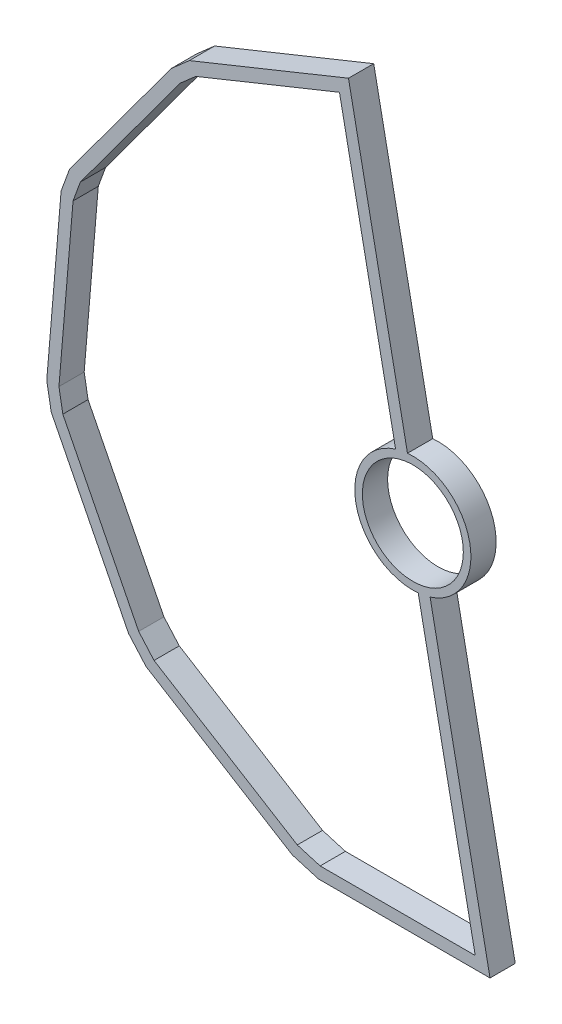
SolidWorks part; units mm, degrees
ref_plane "前视基准面" through (0, 0, 0) normal (0, 0, 1) x (1, 0, 0)
ref_plane "上视基准面" through (0, 0, 0) normal (0, 1, 0) x (1, 0, 0)
ref_plane "右视基准面" through (0, 0, 0) normal (1, 0, 0) x (0, 0, -1)
other "Configuration Table"
sketch "草图1" plane through (0, 0, 0) normal (0, 0, 1) x (1, 0, 0)
  line L12 (10, -352) -> (85, -352)
  line L13 (-85, -352) -> (-10, -352)
  line L14 (-174.7016, -305.0643) -> (-110.8218, -344.3634)
  line L15 (-255.616, -255.2854) -> (-191.7362, -294.5845)
  line L16 (-306.8239, -168.537) -> (-273.0075, -235.4822)
  line L17 (-349.6581, -83.7398) -> (-315.8416, -150.685)
  line L18 (-347.7785, 16.0344) -> (-354.0546, -58.7056)
  line L19 (-339.8288, 110.705) -> (-346.1049, 35.965)
  line L20 (-286.9547, 193.9902) -> (-331.4643, 133.6188)
  line L21 (-230.5758, 270.4605) -> (-275.0855, 210.0892)
  line L22 (-143.2782, 314.1516) -> (-212.8247, 286.053)
  line L23 (-55.1859, 349.7433) -> (-124.7324, 321.6446)
  line L24 (-124.7324, 321.6446) -> (-143.2782, 314.1516)
  line L25 (-212.8247, 286.053) -> (-230.5758, 270.4605)
  line L26 (-275.0855, 210.0892) -> (-286.9547, 193.9902)
  line L27 (-331.4643, 133.6188) -> (-339.8288, 110.705)
  line L28 (-354.0546, -58.7056) -> (-349.6581, -83.7398)
  line L29 (-273.0075, -235.4822) -> (-255.616, -255.2854)
  line L30 (-191.7362, -294.5845) -> (-174.7016, -305.0643)
  line L31 (-110.8218, -344.3634) -> (-85, -352)
  line L32 (-10, -352) -> (10, -352)
  line L33 (85, -352) -> (-55.1859, 349.7433)
  line L34 (-346.1049, 35.965) -> (-347.7785, 16.0344)
  line L35 (-315.8416, -150.685) -> (-306.8239, -168.537)
  line L36 (-138.7829, 303.0254) -> (-206.438, 275.691)
  line L37 (-206.438, 275.691) -> (-221.6847, 262.2984)
  line L38 (-221.6847, 262.2984) -> (-265.4267, 202.9682)
  line L39 (-265.4267, 202.9682) -> (-277.296, 186.8691)
  line L40 (-277.296, 186.8691) -> (-320.7828, 127.8849)
  line L41 (-320.7828, 127.8849) -> (-328.0054, 108.0996)
  line L42 (-328.0054, 108.0996) -> (-334.147, 34.9609)
  line L43 (-334.147, 34.9609) -> (-335.8206, 15.0302)
  line L44 (-335.8206, 15.0302) -> (-341.9666, -58.1608)
  line L45 (-341.9666, -58.1608) -> (-338.1462, -79.9147)
  line L46 (-338.1462, -79.9147) -> (-305.1306, -145.2745)
  line L47 (-305.1306, -145.2745) -> (-296.1129, -163.1265)
  line L48 (-296.1129, -163.1265) -> (-262.9843, -228.7099)
  line L49 (-262.9843, -228.7099) -> (-247.7906, -246.0106)
  line L50 (-247.7906, -246.0106) -> (-185.4483, -284.3638)
  line L51 (-185.4483, -284.3638) -> (-168.4137, -294.8436)
  line L52 (-168.4137, -294.8436) -> (-105.8908, -333.3079)
  line L53 (-105.8908, -333.3079) -> (-83.2627, -340)
  line L54 (-83.2627, -340) -> (-10, -340)
  line L55 (-10, -340) -> (10, -340)
  line L56 (10, -340) -> (70.3657, -340)
  line L57 (70.3657, -340) -> (-64.1167, 333.1926)
  line L58 (-64.1167, 333.1926) -> (-120.2371, 310.5184)
  line L59 (-120.2371, 310.5184) -> (-138.7829, 303.0254)
  dimension "D1" = 12
extrude "凸台-拉伸1" add sketch "草图1" along normal mid plane 25
sketch "草图3" plane through (0, 0, 12.5) normal (0, 0, 1) x (1, 0, 0)
  line L1 (0, 0) -> (8.5631, 0) construction
  line L2 (76.2494, -338.8246) -> (-58.2329, 334.3679)
  line L3 (76.2494, -338.8246) -> (-58.2329, 334.3679) construction
  circle A0 centre (8.5631, 0) radius 50
  dimension "D2" = 100
  dimension "D1" = 6
extrude "切除-拉伸1" cut sketch "草图3" against normal blind 40 contours A0
sketch "草图4" plane through (0, 0, 12.5) normal (0, 0, 1) x (1, 0, 0)
  circle A0 centre (8.5631, 0) radius 50 construction
  circle A1 centre (8.5631, 0) radius 50
  circle A2 centre (8.5631, 0) radius 57.5
  dimension "D1" = 115
extrude "凸台-拉伸2" add sketch "草图4" against normal blind 25
